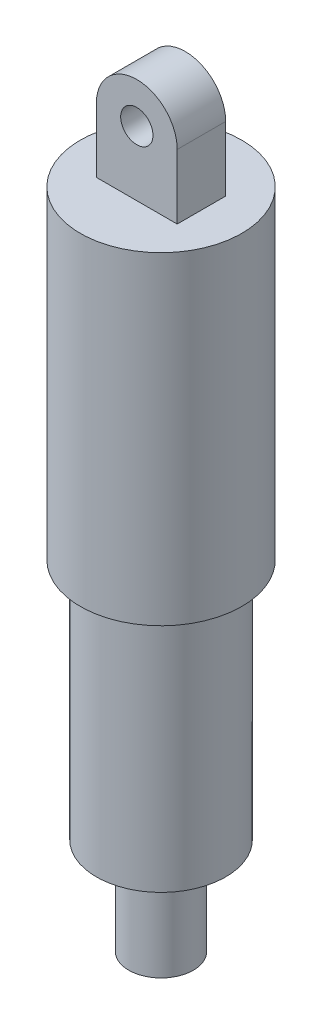
from build123d import *

# Parameters (mm, degrees)
SKETCH2_R           = 10
BOSS_EXTRUDE1_DEPTH = 15


with BuildPart() as part:
    # Sketch1 → Revolve1 (revolve)
    with BuildSketch(Plane.XY, mode=Mode.PRIVATE) as revolve1_sk:
        Polygon((0, 0), (0, 410), (50, 410), (50, 210), (40, 210), (40, 60), (20, 60), (20, 0), align=None)
    revolve(revolve1_sk.sketch.rotate(Axis((0, 0, 0), (0, 1, 0)), 90), axis=Axis((0, 0, 0), (0, 1, 0)))

    # Sketch2 → Boss-Extrude1 (add, symmetric)
    with BuildSketch(Plane.XY):
        with BuildLine():
            Line((-25, 450), (-25, 410))
            Line((-25, 410), (25, 410))
            Line((25, 410), (25, 450))
            ThreePointArc((25, 450), (0, 475), (-25, 450))
        make_face()
        with Locations((0, 450)):
            Circle(SKETCH2_R, mode=Mode.SUBTRACT)
    extrude(amount=BOSS_EXTRUDE1_DEPTH, both=True)


solid = part.part
